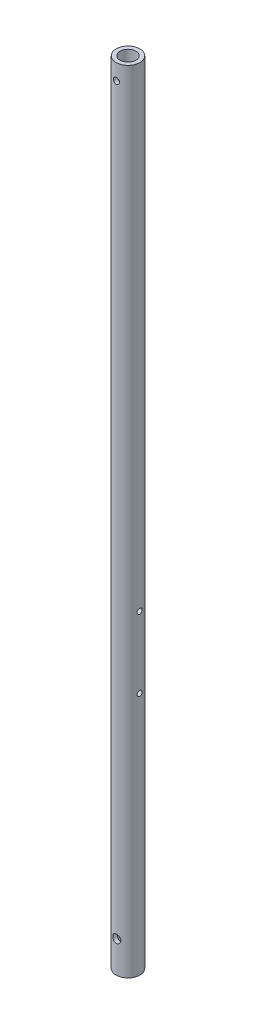
SolidWorks part; units mm, degrees
material "Thornel Mat VMA"
ref_plane "前视基准面" through (0, 0, 0) normal (0, 0, 1) x (1, 0, 0)
ref_plane "上视基准面" through (0, 0, 0) normal (0, 1, 0) x (1, 0, 0)
ref_plane "右视基准面" through (0, 0, 0) normal (1, 0, 0) x (0, 0, -1)
other "Configuration Table"
sketch "草图1" plane through (0, 0, 0) normal (0, 1, 0) x (1, 0, 0)
  circle A0 centre (0, 0) radius 6
  circle A1 centre (0, 0) radius 4
  dimension "D1" = 8
  dimension "D2" = 12
extrude "凸台-拉伸1" add sketch "草图1" along normal blind 400
sketch "草图2" plane through (0, 0, 0) normal (0, 0, 1) x (1, 0, 0)
  line L0 (0, 0) -> (0, 627.0549) construction
  line L3 (6, 400) -> (-6, 400) construction
  line L4 (-6, 0) -> (6, 0) construction
  circle A0 centre (0, 16) radius 2.05
  circle A1 centre (0, 392) radius 1.55
  circle A3 centre (0, 145.5) radius 1.55 construction
  circle A4 centre (0, 160.5) radius 1.3 construction
  circle A5 centre (0, 130.5) radius 1.3 construction
  dimension "D1" = 4.1
  dimension "D2" = 3.1
  dimension "D3" = 8
  dimension "D4" = 16
  dimension "D6" = 3.1
  dimension "D5" = 129.5
  dimension "D7" = 2.6
  dimension "D8" = 30
  dimension "D9" = 15
extrude "切除-拉伸1" cut sketch "草图2" against normal through all both and the other way through all
sketch "草图3" plane through (0, 0, 0) normal (1, 0, 0) x (0, 0, -1)
  line L0 (0, 0) -> (0, 431.1922) construction
  line L1 (0, 141.5) -> (40.9508, 141.5) construction
  line L3 (-6, 0) -> (6, 0) construction
  circle A0 centre (0, 159.5) radius 1.3
  circle A1 centre (0, 123.5) radius 1.3
  dimension "D2" = 2.6
  dimension "D3" = 18
  dimension "D1" = 141.5
extrude "切除-拉伸2" cut sketch "草图3" against normal through all both and the other way through all
